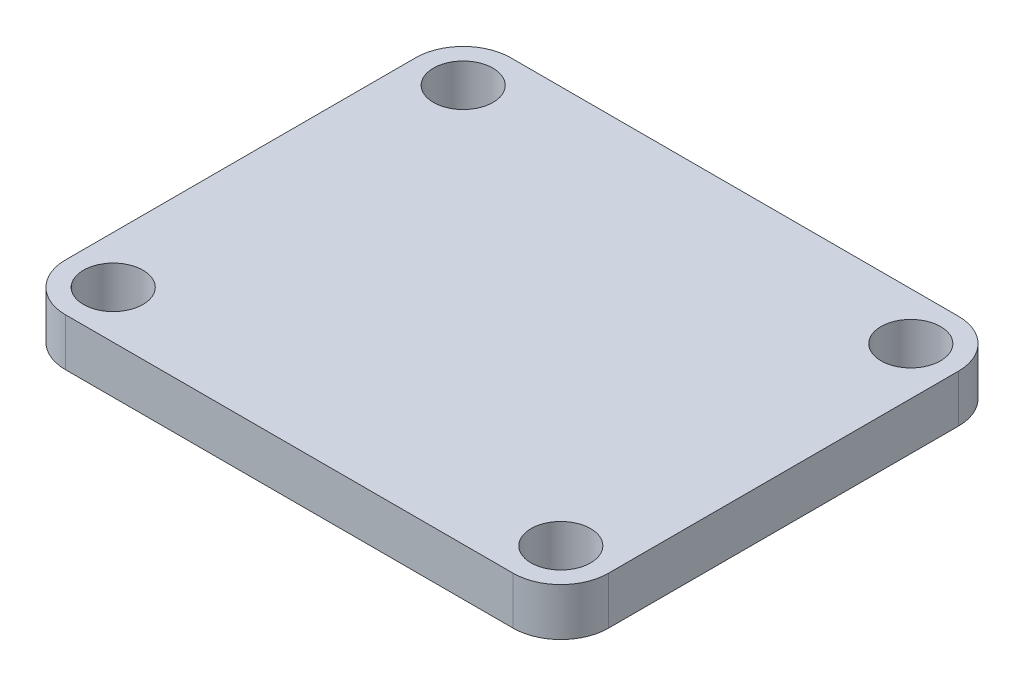
from build123d import *

# Parameters (mm, degrees)
EXTRUDE_THIN1_DEPTH     = 12.7
SKETCH3_W               = 22.8
SKETCH3_H               = 18.7
BOSS_EXTRUDE2_DEPTH     = 2
FILLET1_R               = 2
SKETCH4_R               = 1.25
CUT_EXTRUDE1_DEPTH      = 2
CUT_EXTRUDE2_DEPTH      = 61.42253709
CUT_EXTRUDE2_DEPTH_BACK = 61.42253709
SKETCH5_R               = 2.75
SKETCH6_R               = 1.25
CUT_EXTRUDE3_DEPTH      = 10
CUT_EXTRUDE4_DEPTH      = 131.301684531
CUT_EXTRUDE4_DEPTH_BACK = 131.301684531
SKETCH7_W               = 21.210036283
SKETCH7_H               = 32.49756926


with BuildPart() as part:
    # Sketch1 → Extrude-Thin1 (new body)
    with BuildSketch(Plane.XY):
        Polygon((51.165574182, 84.975681723), (42.185318061, 93.955937844), (42.185318061, 113.634045339), (40.185318061, 113.634045339), (40.185318061, 93.127510719), (49.75136062, 83.561468161), align=None)
    extrude(amount=-EXTRUDE_THIN1_DEPTH)

    # Sketch5 → Cut-Extrude2 (cut, two sides: drawn at the far end of the back side and taken through both)
    with BuildSketch(Plane(origin=(68.070627953, 68.070627953, 0), x_dir=(0, 0, -1), z_dir=(0.7071067811865513, 0.7071067811865437, 0)).offset(-CUT_EXTRUDE2_DEPTH_BACK)):
        with Locations(Location((6.35, 30.257356315, 0), (0, 0, 90))):
            Circle(SKETCH5_R)
    extrude(amount=CUT_EXTRUDE2_DEPTH + CUT_EXTRUDE2_DEPTH_BACK, mode=Mode.SUBTRACT)

    # Sketch6 → Cut-Extrude3 (cut)
    with BuildSketch(Plane(origin=(66.65641439, 66.65641439, 0), x_dir=(0, 0, 1), z_dir=(-0.7071067811865513, -0.7071067811865437, 0))):
        with Locations(Location((-10.65, 34.557356315, 0), (0, 0, 270))):
            Circle(SKETCH6_R)
        with Locations(Location((-2.05, 34.557356315, 0), (0, 0, 270))):
            Circle(SKETCH6_R)
        with Locations(Location((-2.05, 25.957356315, 0), (0, 0, 270))):
            Circle(SKETCH6_R)
        with Locations(Location((-10.65, 25.957356315, 0), (0, 0, 270))):
            Circle(SKETCH6_R)
    extrude(amount=-CUT_EXTRUDE3_DEPTH, mode=Mode.SUBTRACT)

    # Sketch7 → Cut-Extrude4 (cut, two sides: drawn at the far end of the back side and taken through both)
    with BuildSketch(Plane.XY.offset(3).offset(-CUT_EXTRUDE4_DEPTH_BACK)):
        with Locations((44.470427981, 97.385260709)):
            Rectangle(SKETCH7_W, SKETCH7_H)
    extrude(amount=CUT_EXTRUDE4_DEPTH + CUT_EXTRUDE4_DEPTH_BACK, mode=Mode.SUBTRACT)


with BuildPart() as body_2:
    # Sketch3 → Boss-Extrude2 (new body)
    with BuildSketch(Plane(origin=(0, 113.634045339, 0), x_dir=(1, 0, 0), z_dir=(0, 1, 0))):
        with Locations((45.675446122, 6.35)):
            Rectangle(SKETCH3_W, SKETCH3_H)
    extrude(amount=BOSS_EXTRUDE2_DEPTH)

    # Fillet1
    fillet1_edges = [body_2.edges().sort_by_distance(p)[0] for p in [
        (57.075446122, 114.634045339, 3),
        (34.275446122, 114.634045339, 3),
        (34.275446122, 114.634045339, -15.7),
        (57.075446122, 114.634045339, -15.7),
    ]]
    fillet(fillet1_edges, radius=FILLET1_R)

    # Sketch4 → Cut-Extrude1 (cut)
    with BuildSketch(Plane(origin=(0, 115.634045339, 0), x_dir=(1, 0, 0), z_dir=(0, 1, 0))):
        with Locations(Location((55.075446122, 13.7, 0), (0, 0, 270))):
            Circle(SKETCH4_R)
        with Locations(Location((55.075446122, -1, 0), (0, 0, 270))):
            Circle(SKETCH4_R)
        with Locations(Location((36.275446122, -1, 0), (0, 0, 270))):
            Circle(SKETCH4_R)
        with Locations(Location((36.275446122, 13.7, 0), (0, 0, 270))):
            Circle(SKETCH4_R)
    extrude(amount=-CUT_EXTRUDE1_DEPTH, mode=Mode.SUBTRACT)


solid = body_2.part
